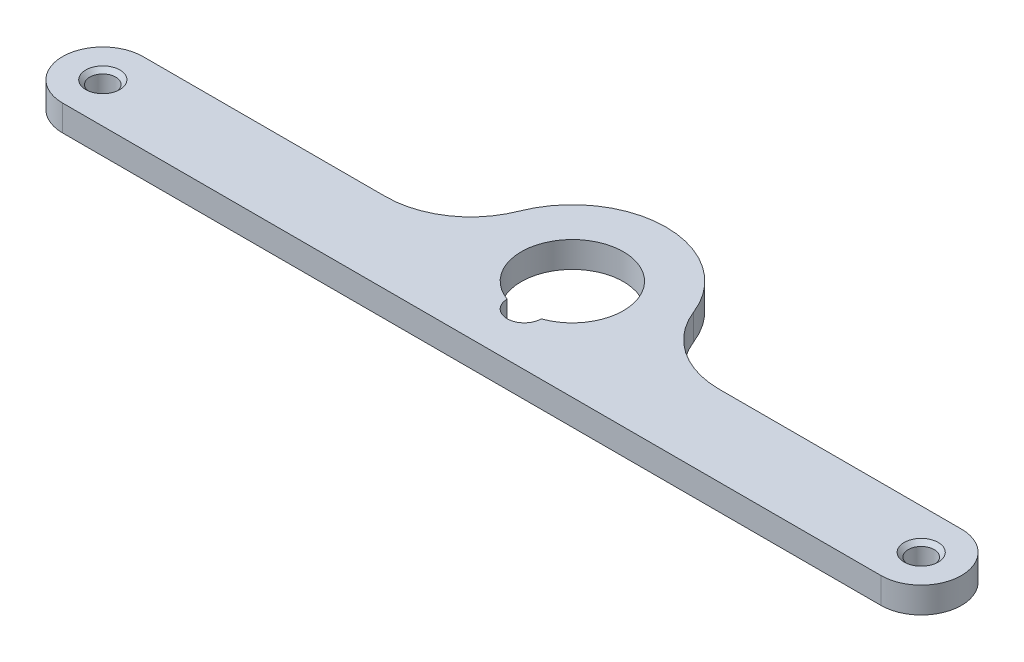
SolidWorks part; units mm, degrees
material "Stainless Steel (ferritic)"
ref_plane "Front" through (0, 0, 0) normal (0, 0, 1) x (1, 0, 0)
ref_plane "Top" through (0, 0, 0) normal (0, 1, 0) x (1, 0, 0)
ref_plane "Right" through (0, 0, 0) normal (1, 0, 0) x (0, 0, -1)
sketch "Sketch1" plane through (0, 0, 0) normal (0, 1, 0) x (1, 0, 0)
  line L0 (-76.2, -18.7325) -> (76.2, -18.7325)
  line L1 (-76.2, -3.7465) -> (-31.0394, -3.7465)
  line L3 (31.0394, -3.7465) -> (76.2, -3.7465)
  arc A0 (3.175, -8.9668) -> (-3.175, -8.9668) centre (0, 0) ccw
  arc A1 (16.2531, 6.3508) -> (-16.2531, 6.3508) centre (0, 0) ccw
  arc A2 (-76.2, -3.7465) -> (-76.2, -18.7325) centre (-76.2, -11.2395) ccw
  arc A3 (76.2, -18.7325) -> (76.2, -3.7465) centre (76.2, -11.2395) ccw
  circle A4 centre (76.2, -11.2395) radius 2.413
  circle A5 centre (-76.2, -11.2395) radius 2.413
  arc A6 (-31.0394, -3.7465) -> (-16.2531, 6.3508) centre (-31.0394, 12.1285) ccw
  arc A7 (31.0394, -3.7465) -> (16.2531, 6.3508) centre (31.0394, 12.1285) cw
  arc A8 (-3.175, -8.9668) -> (3.175, -8.9668) centre (0, -8.9535) ccw
  point P1 (0, 0)
  dimension "D1" = 76.2
  dimension "D3" = 19.0246
  dimension "D4" = 7.9375
  dimension "D5" = 4.826
  dimension "D6" = 14.986
  dimension "D7" = 18.7325
  dimension "D2" = 76.2
  dimension "D8" = 15.875
  dimension "D9" = 6.35
  dimension "D10" = 8.9535
extrude "Boss-Extrude1" add sketch "Sketch1" along normal mid plane 4.826
chamfer "Chamfer1" distance 0.762 angle 45 4 edges at (76.2, -2.413, 13.6525) (76.2, 2.413, 13.6525) (-76.2, -2.413, 13.6525) (-76.2, 2.413, 13.6525)
